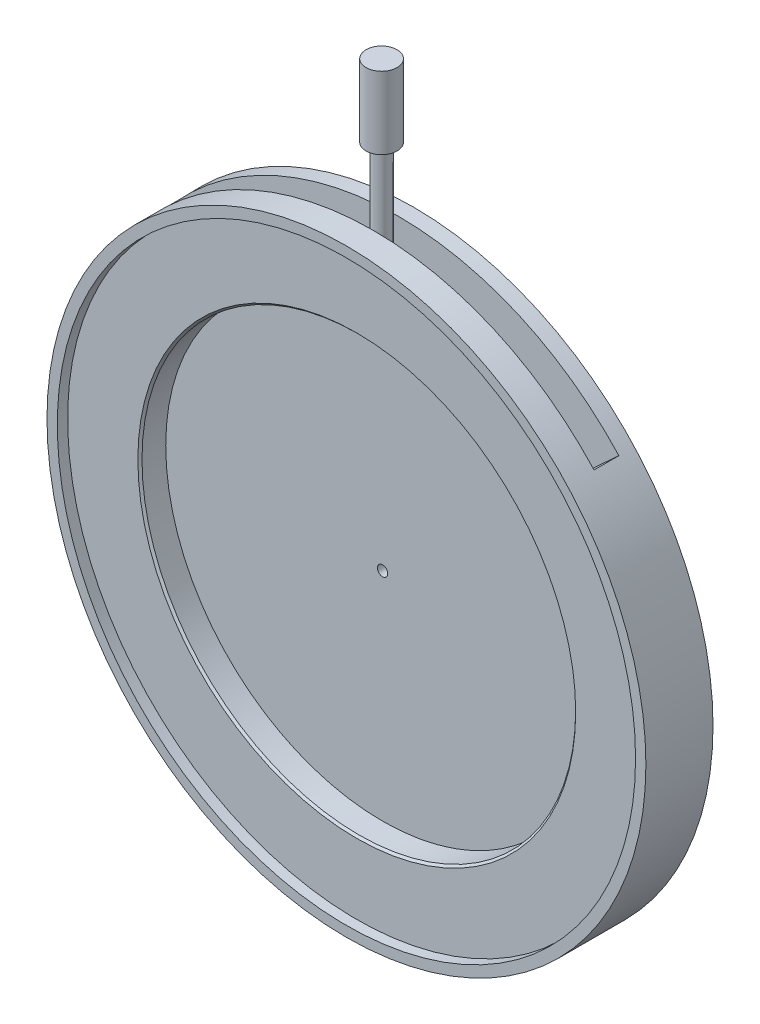
from build123d import *

# Parameters (mm, degrees)
SKETCH_1_R          = 29
SKETCH_1_R_2        = 21
EXTRUDE_1_DEPTH     = 6.5
SKETCH_7_R          = 28
CUT_EXTRUDE_5_DEPTH = 1
CUT_EXTRUDE_START   = -1.5
CUT_EXTRUDE_6_DEPTH = 2.4
MOVE_FACE_1_BY      = 5
EXTRUDE_START       = -3.5
SKETCH_11_R         = 22.5
SKETCH_11_R_2       = 0.5
EXTRUDE_2_DEPTH     = 1
CHAMFER_1_SIZE      = 0.2


with BuildPart() as part:
    # 草图1 → 凸台-拉伸1 (new body)
    with BuildSketch(Plane.XY):
        with Locations(Location((0, 0, 0), (0, 0, 180))):
            Circle(SKETCH_1_R)
        with Locations(Location((0, 0, 0), (0, 0, 180))):
            Circle(SKETCH_1_R_2, mode=Mode.SUBTRACT)
    extrude(amount=EXTRUDE_1_DEPTH)

    # 草图7 → 切除-拉伸5 (cut)
    with BuildSketch(Plane.XY.offset(6.5)):
        Circle(SKETCH_7_R)
    extrude(amount=-CUT_EXTRUDE_5_DEPTH, mode=Mode.SUBTRACT)

    # 草图9 → 切除-拉伸6 (cut)
    with BuildSketch(Plane(origin=(0, 0, 0), x_dir=(-1, 0, 0), z_dir=(0, 0, -1)).offset(CUT_EXTRUDE_START)):
        with BuildLine():
            Line((-18.43193342, 16.88975519), (-21.381042767, 19.592116021))
            ThreePointArc((-21.381042767, 19.592116021), (0, 29), (21.381042767, 19.592116021))
            Line((21.381042767, 19.592116021), (18.43193342, 16.88975519))
            ThreePointArc((18.43193342, 16.88975519), (0, 25), (-18.43193342, 16.88975519))
        make_face()
    extrude(amount=-CUT_EXTRUDE_6_DEPTH, mode=Mode.SUBTRACT)

    # 倒角1
    chamfer_1_edges = [part.edges().sort_by_distance(p)[0] for p in [
        (21, 0, 5.5),
    ]]
    chamfer(chamfer_1_edges, length=CHAMFER_1_SIZE)


with BuildPart() as body_2:
    # 草图10 → 旋转4 (revolve)
    with BuildSketch(Plane(origin=(0, 0, 0), x_dir=(0, 0, -1), z_dir=(1, 0, 0))):
        Polygon((-3.096715261, 43), (-1.596715261, 43), (-1.596715261, 36), (-2.296715261, 36), (-2.296715261, 29), (-3.096715261, 29), align=None)
    revolve(axis=Axis((0, 29, 3.096715261), (0, 1, 0)))

    # Move Face 1: a face moved outward by 5.0
    extrude(body_2.faces().sort_by_distance((0, 29, 3.096715261))[0], amount=MOVE_FACE_1_BY, dir=(0, -1, 0))


with BuildPart() as body_3:
    # 草图11 → 凸台-拉伸2 (new body)
    with BuildSketch(Plane.XY.offset(6.5).offset(EXTRUDE_START)):
        Circle(SKETCH_11_R)
        Circle(SKETCH_11_R_2, mode=Mode.SUBTRACT)
    extrude(amount=-EXTRUDE_2_DEPTH)


solid = Compound([part.part, body_2.part, body_3.part])
